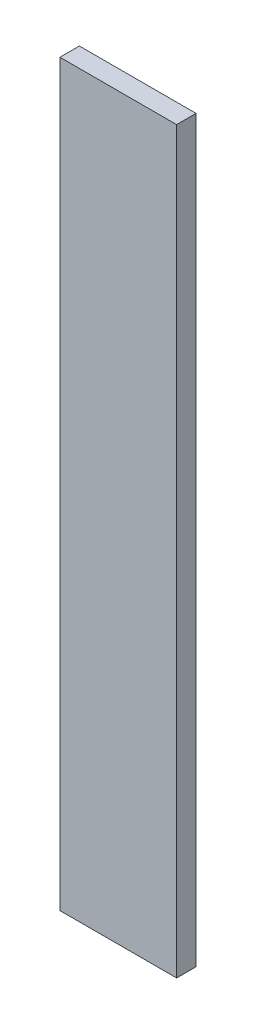
from build123d import *

# Parameters (mm, degrees)
SKETCH_1_W      = 60
SKETCH_1_H      = 380
EXTRUDE_1_DEPTH = 10


with BuildPart() as part:
    # 草图1 → 凸台-拉伸1 (new body)
    with BuildSketch(Plane.XY):
        Rectangle(SKETCH_1_W, SKETCH_1_H)
    extrude(amount=EXTRUDE_1_DEPTH)


solid = part.part
